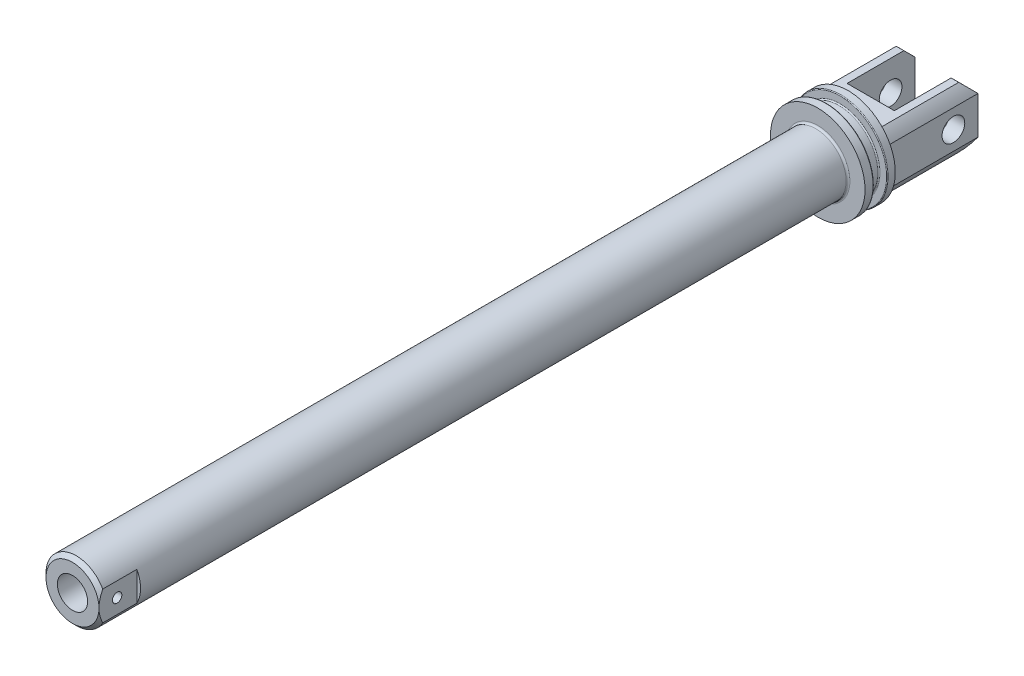
SolidWorks part; units mm, degrees
ref_plane "Front Plane" through (0, 0, 0) normal (0, 0, 1) x (1, 0, 0)
ref_plane "Top Plane" through (0, 0, 0) normal (0, 1, 0) x (1, 0, 0)
ref_plane "Right Plane" through (0, 0, 0) normal (1, 0, 0) x (0, 0, -1)
sketch "Sketch1" plane through (0, 0, 0) normal (0, 0, 1) x (1, 0, 0)
  circle A0 centre (0, 0) radius 8
extrude "Boss-Extrude1" add sketch "Sketch1" along normal blind 197
sketch "Sketch2" plane through (0, 0, 0) normal (0, 0, -1) x (-1, 0, 0)
  circle A0 centre (0, 0) radius 12.5
extrude "Boss-Extrude2" add sketch "Sketch2" along normal blind 8
sketch "Sketch3" plane through (0, 0, 0) normal (0, 1, 0) x (1, 0, 0)
  line L0 (-12.5, 8) -> (-12.5, 0) construction
  line L1 (-12.5, 5.9) -> (-10.25, 5.9)
  line L2 (-12.5, 5.9) -> (-12.5, 2.3)
  line L3 (-12.5, 2.3) -> (-10.25, 2.3)
  line L4 (-10.25, 5.9) -> (-10.25, 2.3)
  line L5 (12.5, 8) -> (-12.5, 8) construction
  line L6 (0, 10.0082) -> (0, -3.7228) construction
  dimension "D1" = 3.6
  dimension "D2" = 2.1
  dimension "D3" = 2.25
revolve "Cut-Revolve1" cut sketch "Sketch3" angle 360 about L6
sketch "Sketch8" plane through (0, 0, -8) normal (0, 0, -1) x (-1, 0, 0)
  circle A0 centre (0, 0) radius 11.5
extrude "Boss-Extrude4" add sketch "Sketch8" along normal blind 24
sketch "Sketch10" plane through (0, 0, 0) normal (0, 1, 0) x (1, 0, 0)
  line L0 (0, 37.7371) -> (0, 5.0633) construction
  line L1 (11.5, 32) -> (-11.5, 32) construction
  line L2 (-6.25, 35.6058) -> (6.25, 35.6058)
  line L3 (-6.25, 35.6058) -> (-6.25, 14)
  line L4 (-6.25, 14) -> (6.25, 14)
  line L5 (6.25, 35.6058) -> (6.25, 14)
  line L6 (-6.25, 35.6058) -> (6.25, 14) construction
  line L7 (-6.25, 14) -> (6.25, 35.6058) construction
  point P3 (0, 24.8029)
  dimension "D1" = 18
  dimension "D2" = 12.5
extrude "Cut-Extrude1" cut sketch "Sketch10" against normal through all both and the other way through all
sketch "Sketch13" plane through (0, 0, -32) normal (0, 0, -1) x (-1, 0, 0)
  line L0 (10.3562, -5) -> (10.3562, 5)
  line L9 (11, 5) -> (10.3562, 4.7073) construction
  line L10 (10.4692, -4.7587) -> (10.3562, -4.7073) construction
  line L11 (-10.3562, -5) -> (-10.3562, 5)
  arc A0 (-10.3562, 5) -> (-10.3562, -5) centre (0, 0) ccw
  arc A1 (10.3562, -5) -> (10.3562, 5) centre (0, 0) ccw
  point P0 (0, 0)
  point P1 (0, 0)
sketch "Sketch11" plane through (0, -11.5, -32) normal (-1, 0, 0) x (0, 0, -1)
  line L1 (-32, -11.5) -> (13.2543, -11.5) construction
  line L7 (1.4984, -3.5) -> (-24, -19.5) construction
  line L8 (1.4984, -19.5) -> (-24, -3.5) construction
  line L9 (0.011, -16.5) -> (-3, -19.5)
  line L11 (-24, -19.5) -> (-24, -26.3966)
  line L12 (-24, -26.3966) -> (1.4984, -26.3966)
  line L13 (1.4984, -19.5) -> (1.4984, -26.3966)
  line L15 (-24, -3.5) -> (-24, 3.3597)
  line L16 (-24, 3.3597) -> (2.7695, 3.3597)
  line L17 (2.7695, -3.5) -> (2.7695, 3.3597)
  line L18 (0, -21.1534) -> (0, -1.8466) construction
  line L19 (1.4984, -19.5) -> (0.011, -19.5)
  line L20 (0.011, -19.5) -> (0.011, -16.5)
  line L21 (-3, -19.5) -> (-24, -19.5)
  line L22 (-3, -3.5) -> (-24, -3.5)
  line L23 (0.011, -6.5) -> (-3, -3.5)
  line L24 (0.011, -3.5) -> (0.011, -6.5)
  line L25 (1.4984, -3.5) -> (0.011, -3.5)
  line L26 (1.4984, -3.5) -> (2.7695, -3.5)
  point P0 (-11.2508, -11.5)
  dimension "D1" = 3
  dimension "D2" = 16
  dimension "D3" = 3
extrude "Cut-Extrude3" cut sketch "Sketch11" against normal through all both and the other way through all
extrude "Cut-Extrude5" cut sketch "Sketch13" against normal blind 24
fillet "Fillet1" radius 0.5 1 edges at (8, 0, 0)
fillet "Fillet2" radius 0.2 2 edges at (-12.5, 0, -5.9) (-12.5, 0, -2.3)
fillet "Fillet3" radius 0.3 2 edges at (-10.25, 0, -2.3) (-10.25, 0, -5.9)
chamfer "Chamfer3" distance 1 angle 45 1 edges at (8, 0, 197)
sketch "Sketch15" plane through (0, 8, 0) normal (0, 1, 0) x (1, 0, 0)
  line L0 (8, -196) -> (8, -0.5) construction
  line L1 (-7, -187) -> (-9.1993, -187)
  line L2 (-7, -187) -> (-7, -195)
  line L3 (-7, -195) -> (-9.1993, -195)
  line L4 (-9.1993, -187) -> (-9.1993, -195)
  line L5 (-8.5, -153.05) -> (-9.4702, -153.05)
  line L6 (-6, -155.55) -> (-6, -175.45)
  line L7 (-8.5, -177.95) -> (-9.4702, -177.95)
  line L8 (-9.4702, -153.05) -> (-9.4702, -177.95)
  line L9 (-8, -197) -> (8, -197) construction
  line L10 (9.8801, -187) -> (7, -187)
  line L11 (9.8801, -187) -> (9.8801, -197)
  line L12 (9.8801, -197) -> (7, -197)
  line L13 (7, -187) -> (7, -197)
  line L14 (-8, -0.5) -> (-8, -196) construction
  arc A0 (-8.5, -177.95) -> (-6, -175.45) centre (-8.5, -175.45) ccw
  arc A1 (-8.5, -153.05) -> (-6, -155.55) centre (-8.5, -155.55) cw
  dimension "D10" = 2.5
  dimension "D1" = 24.9
  dimension "D2" = 8
  dimension "D3" = 14
  dimension "D4" = 10
  dimension "D5" = 10
  dimension "D6" = 0
  dimension "D7" = 14
  dimension "D8" = 1
  dimension "D9" = 19.05
extrude "Cut-Extrude7" cut sketch "Sketch15" against normal through all both and the other way through all
sketch "Sketch14" plane through (10.3562, 0, 0) normal (1, 0, 0) x (0, 0, -1)
  line L0 (32, -5) -> (32, 5) construction
  circle A0 centre (25.5, 0) radius 3
  dimension "D1" = 6.5
extrude "Cut-Extrude6" cut sketch "Sketch14" against normal blind 24
sketch "Sketch16" plane through (7, 0, 0) normal (1, 0, 0) x (0, 0, -1)
  line L0 (-196, -8) -> (-0.5, -8) construction
  line L1 (-197, 7) -> (-197, -7) construction
  circle A0 centre (-192.2, 0) radius 0.6474
  dimension "D1" = 8
  dimension "D2" = 4.8
hole_wizard "Hole2" positions "Sketch18" profile "Sketch19" legacy
sketch "Sketch18" plane through (0, 0, 197) normal (0, 0, 1) x (1, 0, 0)
  point P0 (0, 0)
sketch "Sketch19" plane through (0, 0, 197) normal (1, 0, 0) x (0, -1, 0)
  line L0 (0, 0) -> (0, 7.5)
  line L1 (0, 7.5) -> (4, 7.5)
  line L2 (4, 7.5) -> (4, 0)
  line L3 (4, 0) -> (0, 0)
  line L4 (0, 110) -> (0, -10) construction
  dimension "直径" = 8
  dimension "深度" = 7.5
hole_wizard "M6 Tapped Hole1" positions "Sketch20" profile "Sketch21" tap size "M6" standard "GB"
sketch "Sketch20" plane through (0, 0, 197) normal (0, 0, 1) x (1, 0, 0)
  point P0 (0, 0)
sketch "Sketch21" plane through (0, 0, 197) normal (1, 0, 0) x (0, -1, 0)
  line L0 (0, 0) -> (0, 19.5022)
  line L1 (0, 19.5022) -> (2.5, 18)
  line L2 (2.5, 18) -> (2.5, 0)
  line L5 (2.5, 0) -> (0, 0)
  line L10 (0, 19.5022) -> (-2.5, 18) construction
  line L11 (0, -6.35) -> (0, 107.95) construction
  dimension "螺纹孔钻头直径" = 5
  dimension "螺纹孔钻头深度" = 18
  dimension "导头角度" = 118
cosmetic thread "Cosmetic Thread1" parameters "D1"=12, "D2"=6
hole_wizard "M3 Tapped Hole1" positions "Sketch22" profile "Sketch23" tap size "M3" standard "GB"
sketch "Sketch22" plane through (7, 0, 0) normal (1, 0, 0) x (0, 0, -1)
  point P0 (-192.2, 0)
sketch "Sketch23" plane through (7, 0, 192.2) normal (0, 1, 0) x (0, 0, -1)
  line L0 (0, 0) -> (0, 8.2511)
  line L1 (0, 8.2511) -> (1.25, 7.5)
  line L2 (1.25, 7.5) -> (1.25, 0)
  line L5 (1.25, 0) -> (0, 0)
  line L10 (0, 8.2511) -> (-1.25, 7.5) construction
  line L11 (0, -6.35) -> (0, 107.95) construction
  dimension "螺纹孔钻头直径" = 2.5
  dimension "螺纹孔钻头深度" = 7.5
  dimension "导头角度" = 118
cosmetic thread "Cosmetic Thread2" parameters "D1"=3.2003, "D2"=3
